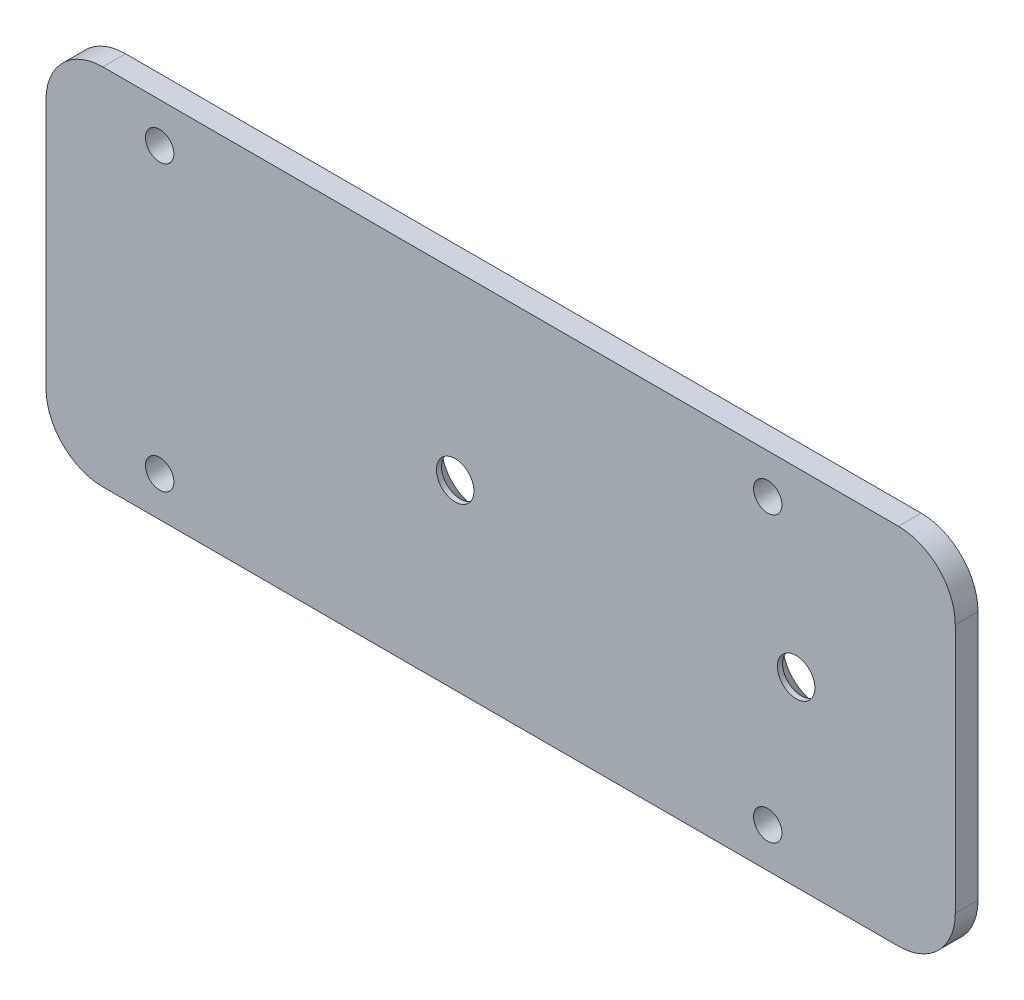
from build123d import *

# Parameters (mm, degrees)
SKETCH_1_W               = 160
SKETCH_1_H               = 64
EXTRUDE_1_DEPTH          = 4
FILLET_1_R               = 10
HOLE_WIZARD_M6_1_D       = 5
HOLE_WIZARD_2_AT_2_COUNT = 2
HOLE_WIZARD_2_AT_2_PITCH = 60


with BuildPart() as part:
    # 草图1 → 凸台-拉伸1 (new body)
    with BuildSketch(Plane.XY):
        Rectangle(SKETCH_1_W, SKETCH_1_H)
    extrude(amount=EXTRUDE_1_DEPTH)

    # 圆角1
    fillet_1_edges = [part.edges().sort_by_distance(p)[0] for p in [
        (80, -32, 2),
        (-80, -32, 2),
        (-80, 32, 2),
        (80, 32, 2),
    ]]
    fillet(fillet_1_edges, radius=FILLET_1_R)

    # M6 螺纹孔1 (through all)
    with Locations(Plane.XY.offset(4)):
        with Locations((-60, 25), (-60, -25), (47, 25), (47, -25)):
            Hole(HOLE_WIZARD_M6_1_D / 2)

    # 草图6 → 打孔尺寸(%根据)内六角花形半沉头螺钉的类型2 (revolve, cut)
    with BuildSketch(Plane.YZ.offset(52)):
        Polygon((0, 0), (0, 4), (3.3, 4), (3.3, 3.1), (6.4, 0), align=None)
    hole_wizard_2 = revolve(axis=Axis((52, 0, -6.35), (0, 0, 1)), mode=Mode.SUBTRACT)

    # 打孔尺寸(%根据)内六角花形半沉头螺钉的类型2 at 2: 打孔尺寸(%根据)内六角花形半沉头螺钉的类型2 ×2
    with Locations(*[(-i * HOLE_WIZARD_2_AT_2_PITCH, 0, 0) for i in range(1, HOLE_WIZARD_2_AT_2_COUNT)]):
        add(hole_wizard_2, mode=Mode.SUBTRACT)


solid = part.part
